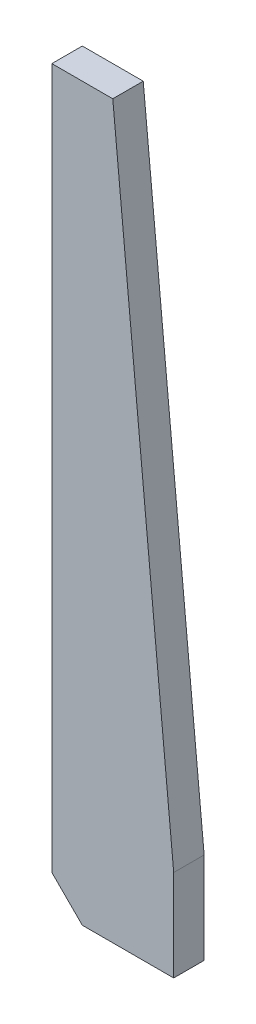
SolidWorks part; units mm, degrees
material "Q235-A"
ref_plane "前视基准面" through (0, 0, 0) normal (0, 0, 1) x (1, 0, 0)
ref_plane "上视基准面" through (0, 0, 0) normal (0, 1, 0) x (1, 0, 0)
ref_plane "右视基准面" through (0, 0, 0) normal (1, 0, 0) x (0, 0, -1)
sketch "草图1" plane through (0, 0, 0) normal (0, 0, 1) x (1, 0, 0)
  line L0 (0, 0) -> (0, 120)
  line L1 (0, 120) -> (10, 120)
  line L2 (10, 120) -> (20, 15)
  line L3 (20, 15) -> (20, 0)
  line L4 (20, 0) -> (0, 0)
  dimension "D1" = 20
  dimension "D2" = 120
  dimension "D3" = 10
  dimension "D4" = 15
extrude "凸台-拉伸1" add sketch "草图1" along normal blind 5
chamfer "倒角1" distance 5 angle 45 1 edges at (0, 0, 2.5)
